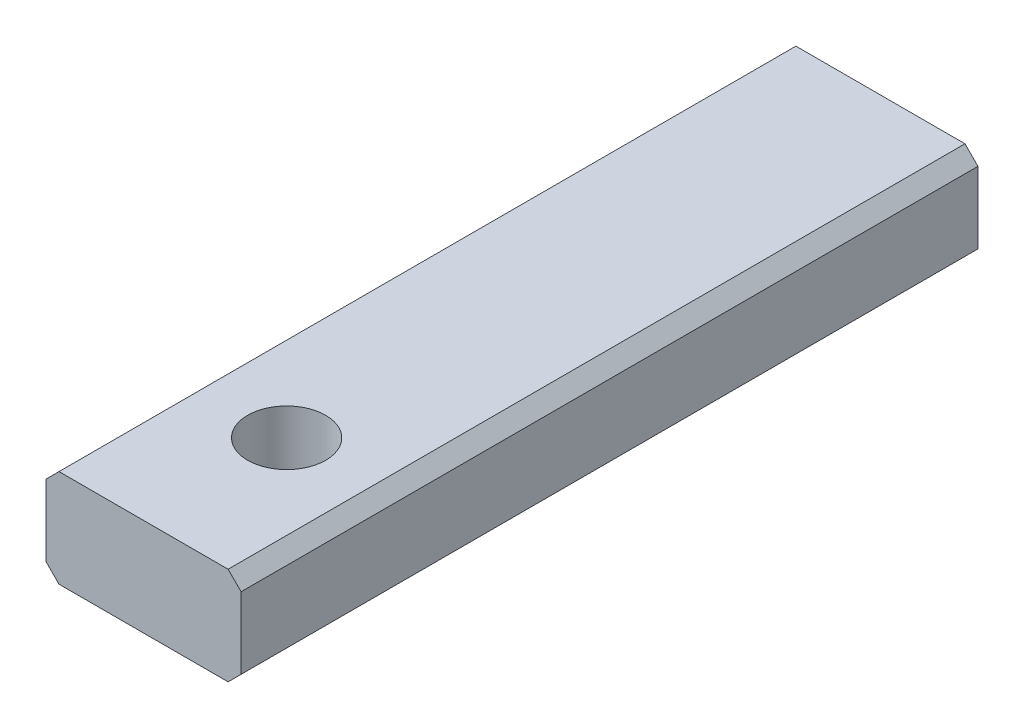
from build123d import *

# Parameters (mm, degrees)
BOSS_EXTRUDE1_DEPTH          = 113.3
SKETCH2_R                    = 6
CUT_EXTRUDE1_DEPTH           = 110
M8_TAPPED_HOLE_1_D           = 6.8
M8_TAPPED_HOLE_1_DEPTH       = 17
M8_TAPPED_HOLE_1_CSINK_D     = 8.05
M8_TAPPED_HOLE_1_CSINK_ANGLE = 90
M8_TAPPED_HOLE_1_TIP         = 2.042926105


with BuildPart() as part:
    # Sketch1 → Boss-Extrude1 (new body)
    with BuildSketch(Plane.XY):
        Polygon((-113, 41), (-87, 41), (-85, 39), (-85, 28), (-87, 26), (-113, 26), (-115, 28), (-115, 39), align=None)
    extrude(amount=BOSS_EXTRUDE1_DEPTH)

    # Sketch2 → Cut-Extrude1 (cut)
    with BuildSketch(Plane(origin=(0, 26, 0), x_dir=(-1, 0, 0), z_dir=(0, -1, 0))):
        with Locations(Location((100, -91.3, 0), (0, 0, 90))):
            Circle(SKETCH2_R)
    extrude(amount=-CUT_EXTRUDE1_DEPTH, mode=Mode.SUBTRACT)

    # M8 Tapped Hole 1
    with Locations(Plane(origin=(0, 0, 0), x_dir=(-1, 0, 0), z_dir=(0, 0, -1))):
        with Locations((100, 33.5)):
            CounterSinkHole(M8_TAPPED_HOLE_1_D / 2, M8_TAPPED_HOLE_1_CSINK_D / 2, depth=M8_TAPPED_HOLE_1_DEPTH, counter_sink_angle=M8_TAPPED_HOLE_1_CSINK_ANGLE)
            with Locations((0, 0, -(M8_TAPPED_HOLE_1_DEPTH + M8_TAPPED_HOLE_1_TIP / 2))):  # 118° drill point
                Cone(0, M8_TAPPED_HOLE_1_D / 2, M8_TAPPED_HOLE_1_TIP, mode=Mode.SUBTRACT)


solid = part.part
